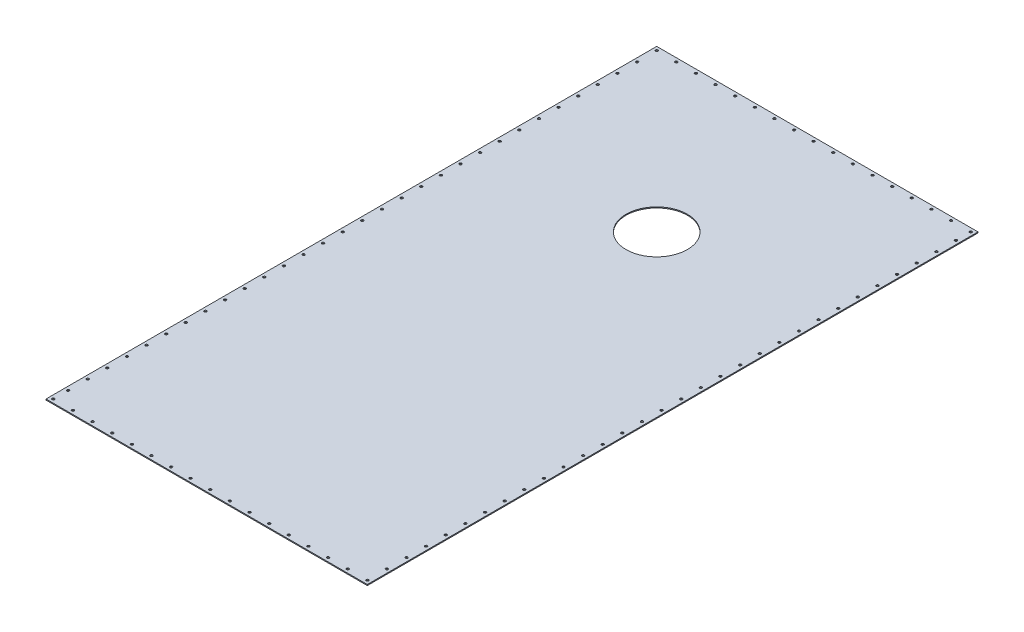
from build123d import *

# Parameters (mm, degrees)
SKETCH_1_W               = 1310
SKETCH_1_H               = 2490
EXTRUDE_1_DEPTH          = 4
PATTERN_LINEAR_1_COUNT   = 17
PATTERN_LINEAR_1_PITCH   = 80
PATTERN_CIRCULAR_1_COUNT = 2
SKETCH_4_R               = 125
CUT_EXTRUDE_1_DEPTH      = 2814.577082648
PATTERN_LINEAR_2_COUNT   = 30
PATTERN_LINEAR_2_PITCH   = 80
PATTERN_CIRCULAR_2_COUNT = 2


with BuildPart() as part:
    # 草图1 → 凸台-拉伸1 (new body)
    with BuildSketch(Plane(origin=(0, 0, 0), x_dir=(1, 0, 0), z_dir=(0, 1, 0))):
        with Locations((655, 1245)):
            Rectangle(SKETCH_1_W, SKETCH_1_H)
    extrude(amount=EXTRUDE_1_DEPTH)

    # 草图2 → Ø10.0 (10) 直径孔1 (revolve, cut)
    with BuildSketch(Plane(origin=(15, 4, -15), x_dir=(0, 0, 1), z_dir=(1, 0, 0))):
        Polygon((0, 0), (0, 13.004303095), (5, 10), (5, 0), align=None)
    hole_wizard_10_0_10_1 = revolve(axis=Axis((15, 10.35, -15), (0, -1, 0)), mode=Mode.SUBTRACT)

    # 阵列(线性)1: Ø10.0 (10) 直径孔1 ×17
    with Locations(*[(i * PATTERN_LINEAR_1_PITCH, 0, 0) for i in range(1, PATTERN_LINEAR_1_COUNT)]):
        add(hole_wizard_10_0_10_1, mode=Mode.SUBTRACT)

    # 阵列(圆周)1: Ø10.0 (10) 直径孔1 ×2 about axis
    pattern_circular_1_axis = Axis((655, 0, -1245), (0, 1, 0))
    for i in range(1, PATTERN_CIRCULAR_1_COUNT):
        add(hole_wizard_10_0_10_1.rotate(pattern_circular_1_axis, i * 360 / PATTERN_CIRCULAR_1_COUNT), mode=Mode.SUBTRACT)

    # 阵列(圆周)1 copy 1 sketch → 阵列(圆周)1 copy 1 (revolve, cut)
    with BuildSketch(Plane(origin=(1215, 4, -2475), x_dir=(0, 0, -1), z_dir=(-1, 0, 0))):
        Polygon((0, 0), (0, 13.004303095), (5, 10), (5, 0), align=None)
    revolve(axis=Axis((1215, 10.35, -2475), (0, -1, 0)), mode=Mode.SUBTRACT)

    # 阵列(圆周)1 copy 2 sketch → 阵列(圆周)1 copy 2 (revolve, cut)
    with BuildSketch(Plane(origin=(1135, 4, -2475), x_dir=(0, 0, -1), z_dir=(-1, 0, 0))):
        Polygon((0, 0), (0, 13.004303095), (5, 10), (5, 0), align=None)
    revolve(axis=Axis((1135, 10.35, -2475), (0, -1, 0)), mode=Mode.SUBTRACT)

    # 阵列(圆周)1 copy 3 sketch → 阵列(圆周)1 copy 3 (revolve, cut)
    with BuildSketch(Plane(origin=(1055, 4, -2475), x_dir=(0, 0, -1), z_dir=(-1, 0, 0))):
        Polygon((0, 0), (0, 13.004303095), (5, 10), (5, 0), align=None)
    revolve(axis=Axis((1055, 10.35, -2475), (0, -1, 0)), mode=Mode.SUBTRACT)

    # 阵列(圆周)1 copy 4 sketch → 阵列(圆周)1 copy 4 (revolve, cut)
    with BuildSketch(Plane(origin=(975, 4, -2475), x_dir=(0, 0, -1), z_dir=(-1, 0, 0))):
        Polygon((0, 0), (0, 13.004303095), (5, 10), (5, 0), align=None)
    revolve(axis=Axis((975, 10.35, -2475), (0, -1, 0)), mode=Mode.SUBTRACT)

    # 阵列(圆周)1 copy 5 sketch → 阵列(圆周)1 copy 5 (revolve, cut)
    with BuildSketch(Plane(origin=(895, 4, -2475), x_dir=(0, 0, -1), z_dir=(-1, 0, 0))):
        Polygon((0, 0), (0, 13.004303095), (5, 10), (5, 0), align=None)
    revolve(axis=Axis((895, 10.35, -2475), (0, -1, 0)), mode=Mode.SUBTRACT)

    # 阵列(圆周)1 copy 6 sketch → 阵列(圆周)1 copy 6 (revolve, cut)
    with BuildSketch(Plane(origin=(815, 4, -2475), x_dir=(0, 0, -1), z_dir=(-1, 0, 0))):
        Polygon((0, 0), (0, 13.004303095), (5, 10), (5, 0), align=None)
    revolve(axis=Axis((815, 10.35, -2475), (0, -1, 0)), mode=Mode.SUBTRACT)

    # 阵列(圆周)1 copy 7 sketch → 阵列(圆周)1 copy 7 (revolve, cut)
    with BuildSketch(Plane(origin=(735, 4, -2475), x_dir=(0, 0, -1), z_dir=(-1, 0, 0))):
        Polygon((0, 0), (0, 13.004303095), (5, 10), (5, 0), align=None)
    revolve(axis=Axis((735, 10.35, -2475), (0, -1, 0)), mode=Mode.SUBTRACT)

    # 阵列(圆周)1 copy 8 sketch → 阵列(圆周)1 copy 8 (revolve, cut)
    with BuildSketch(Plane(origin=(655, 4, -2475), x_dir=(0, 0, -1), z_dir=(-1, 0, 0))):
        Polygon((0, 0), (0, 13.004303095), (5, 10), (5, 0), align=None)
    revolve(axis=Axis((655, 10.35, -2475), (0, -1, 0)), mode=Mode.SUBTRACT)

    # 阵列(圆周)1 copy 9 sketch → 阵列(圆周)1 copy 9 (revolve, cut)
    with BuildSketch(Plane(origin=(575, 4, -2475), x_dir=(0, 0, -1), z_dir=(-1, 0, 0))):
        Polygon((0, 0), (0, 13.004303095), (5, 10), (5, 0), align=None)
    revolve(axis=Axis((575, 10.35, -2475), (0, -1, 0)), mode=Mode.SUBTRACT)

    # 阵列(圆周)1 copy 10 sketch → 阵列(圆周)1 copy 10 (revolve, cut)
    with BuildSketch(Plane(origin=(495, 4, -2475), x_dir=(0, 0, -1), z_dir=(-1, 0, 0))):
        Polygon((0, 0), (0, 13.004303095), (5, 10), (5, 0), align=None)
    revolve(axis=Axis((495, 10.35, -2475), (0, -1, 0)), mode=Mode.SUBTRACT)

    # 阵列(圆周)1 copy 11 sketch → 阵列(圆周)1 copy 11 (revolve, cut)
    with BuildSketch(Plane(origin=(415, 4, -2475), x_dir=(0, 0, -1), z_dir=(-1, 0, 0))):
        Polygon((0, 0), (0, 13.004303095), (5, 10), (5, 0), align=None)
    revolve(axis=Axis((415, 10.35, -2475), (0, -1, 0)), mode=Mode.SUBTRACT)

    # 阵列(圆周)1 copy 12 sketch → 阵列(圆周)1 copy 12 (revolve, cut)
    with BuildSketch(Plane(origin=(335, 4, -2475), x_dir=(0, 0, -1), z_dir=(-1, 0, 0))):
        Polygon((0, 0), (0, 13.004303095), (5, 10), (5, 0), align=None)
    revolve(axis=Axis((335, 10.35, -2475), (0, -1, 0)), mode=Mode.SUBTRACT)

    # 阵列(圆周)1 copy 13 sketch → 阵列(圆周)1 copy 13 (revolve, cut)
    with BuildSketch(Plane(origin=(255, 4, -2475), x_dir=(0, 0, -1), z_dir=(-1, 0, 0))):
        Polygon((0, 0), (0, 13.004303095), (5, 10), (5, 0), align=None)
    revolve(axis=Axis((255, 10.35, -2475), (0, -1, 0)), mode=Mode.SUBTRACT)

    # 阵列(圆周)1 copy 14 sketch → 阵列(圆周)1 copy 14 (revolve, cut)
    with BuildSketch(Plane(origin=(175, 4, -2475), x_dir=(0, 0, -1), z_dir=(-1, 0, 0))):
        Polygon((0, 0), (0, 13.004303095), (5, 10), (5, 0), align=None)
    revolve(axis=Axis((175, 10.35, -2475), (0, -1, 0)), mode=Mode.SUBTRACT)

    # 阵列(圆周)1 copy 15 sketch → 阵列(圆周)1 copy 15 (revolve, cut)
    with BuildSketch(Plane(origin=(95, 4, -2475), x_dir=(0, 0, -1), z_dir=(-1, 0, 0))):
        Polygon((0, 0), (0, 13.004303095), (5, 10), (5, 0), align=None)
    revolve(axis=Axis((95, 10.35, -2475), (0, -1, 0)), mode=Mode.SUBTRACT)

    # 阵列(圆周)1 copy 16 sketch → 阵列(圆周)1 copy 16 (revolve, cut)
    with BuildSketch(Plane(origin=(15, 4, -2475), x_dir=(0, 0, -1), z_dir=(-1, 0, 0))):
        Polygon((0, 0), (0, 13.004303095), (5, 10), (5, 0), align=None)
    revolve(axis=Axis((15, 10.35, -2475), (0, -1, 0)), mode=Mode.SUBTRACT)

    # 草图4 → 切除-拉伸1 (cut, through all)
    with BuildSketch(Plane(origin=(0, 4, 0), x_dir=(1, 0, 0), z_dir=(0, 1, 0))):
        with Locations(Location((655, 1835, 0), (0, 0, 270))):
            Circle(SKETCH_4_R)
    extrude(amount=-CUT_EXTRUDE_1_DEPTH, mode=Mode.SUBTRACT)

    # 草图5 → Ø10.0 (10) 直径孔2 (revolve, cut)
    with BuildSketch(Plane(origin=(15, 4, -2395), x_dir=(0, 0, 1), z_dir=(1, 0, 0))):
        Polygon((0, 0), (0, 1269.004303095), (5, 1266), (5, 0), align=None)
    hole_wizard_10_0_10_2 = revolve(axis=Axis((15, 10.35, -2395), (0, -1, 0)), mode=Mode.SUBTRACT)

    # 阵列(线性)2: Ø10.0 (10) 直径孔2 ×30
    with Locations(*[(0, 0, i * PATTERN_LINEAR_2_PITCH) for i in range(1, PATTERN_LINEAR_2_COUNT)]):
        add(hole_wizard_10_0_10_2, mode=Mode.SUBTRACT)

    # 阵列(圆周)2: Ø10.0 (10) 直径孔2 ×2 about axis
    pattern_circular_2_axis = Axis((655, 0, -1245), (0, 1, 0))
    for i in range(1, PATTERN_CIRCULAR_2_COUNT):
        add(hole_wizard_10_0_10_2.rotate(pattern_circular_2_axis, i * 360 / PATTERN_CIRCULAR_2_COUNT), mode=Mode.SUBTRACT)

    # 阵列(圆周)2 copy 1 sketch → 阵列(圆周)2 copy 1 (revolve, cut)
    with BuildSketch(Plane(origin=(1295, 4, -175), x_dir=(0, 0, -1), z_dir=(-1, 0, 0))):
        Polygon((0, 0), (0, 1269.004303095), (5, 1266), (5, 0), align=None)
    revolve(axis=Axis((1295, 10.35, -175), (0, -1, 0)), mode=Mode.SUBTRACT)

    # 阵列(圆周)2 copy 2 sketch → 阵列(圆周)2 copy 2 (revolve, cut)
    with BuildSketch(Plane(origin=(1295, 4, -255), x_dir=(0, 0, -1), z_dir=(-1, 0, 0))):
        Polygon((0, 0), (0, 1269.004303095), (5, 1266), (5, 0), align=None)
    revolve(axis=Axis((1295, 10.35, -255), (0, -1, 0)), mode=Mode.SUBTRACT)

    # 阵列(圆周)2 copy 3 sketch → 阵列(圆周)2 copy 3 (revolve, cut)
    with BuildSketch(Plane(origin=(1295, 4, -335), x_dir=(0, 0, -1), z_dir=(-1, 0, 0))):
        Polygon((0, 0), (0, 1269.004303095), (5, 1266), (5, 0), align=None)
    revolve(axis=Axis((1295, 10.35, -335), (0, -1, 0)), mode=Mode.SUBTRACT)

    # 阵列(圆周)2 copy 4 sketch → 阵列(圆周)2 copy 4 (revolve, cut)
    with BuildSketch(Plane(origin=(1295, 4, -415), x_dir=(0, 0, -1), z_dir=(-1, 0, 0))):
        Polygon((0, 0), (0, 1269.004303095), (5, 1266), (5, 0), align=None)
    revolve(axis=Axis((1295, 10.35, -415), (0, -1, 0)), mode=Mode.SUBTRACT)

    # 阵列(圆周)2 copy 5 sketch → 阵列(圆周)2 copy 5 (revolve, cut)
    with BuildSketch(Plane(origin=(1295, 4, -495), x_dir=(0, 0, -1), z_dir=(-1, 0, 0))):
        Polygon((0, 0), (0, 1269.004303095), (5, 1266), (5, 0), align=None)
    revolve(axis=Axis((1295, 10.35, -495), (0, -1, 0)), mode=Mode.SUBTRACT)

    # 阵列(圆周)2 copy 6 sketch → 阵列(圆周)2 copy 6 (revolve, cut)
    with BuildSketch(Plane(origin=(1295, 4, -575), x_dir=(0, 0, -1), z_dir=(-1, 0, 0))):
        Polygon((0, 0), (0, 1269.004303095), (5, 1266), (5, 0), align=None)
    revolve(axis=Axis((1295, 10.35, -575), (0, -1, 0)), mode=Mode.SUBTRACT)

    # 阵列(圆周)2 copy 7 sketch → 阵列(圆周)2 copy 7 (revolve, cut)
    with BuildSketch(Plane(origin=(1295, 4, -655), x_dir=(0, 0, -1), z_dir=(-1, 0, 0))):
        Polygon((0, 0), (0, 1269.004303095), (5, 1266), (5, 0), align=None)
    revolve(axis=Axis((1295, 10.35, -655), (0, -1, 0)), mode=Mode.SUBTRACT)

    # 阵列(圆周)2 copy 8 sketch → 阵列(圆周)2 copy 8 (revolve, cut)
    with BuildSketch(Plane(origin=(1295, 4, -735), x_dir=(0, 0, -1), z_dir=(-1, 0, 0))):
        Polygon((0, 0), (0, 1269.004303095), (5, 1266), (5, 0), align=None)
    revolve(axis=Axis((1295, 10.35, -735), (0, -1, 0)), mode=Mode.SUBTRACT)

    # 阵列(圆周)2 copy 9 sketch → 阵列(圆周)2 copy 9 (revolve, cut)
    with BuildSketch(Plane(origin=(1295, 4, -815), x_dir=(0, 0, -1), z_dir=(-1, 0, 0))):
        Polygon((0, 0), (0, 1269.004303095), (5, 1266), (5, 0), align=None)
    revolve(axis=Axis((1295, 10.35, -815), (0, -1, 0)), mode=Mode.SUBTRACT)

    # 阵列(圆周)2 copy 10 sketch → 阵列(圆周)2 copy 10 (revolve, cut)
    with BuildSketch(Plane(origin=(1295, 4, -895), x_dir=(0, 0, -1), z_dir=(-1, 0, 0))):
        Polygon((0, 0), (0, 1269.004303095), (5, 1266), (5, 0), align=None)
    revolve(axis=Axis((1295, 10.35, -895), (0, -1, 0)), mode=Mode.SUBTRACT)

    # 阵列(圆周)2 copy 11 sketch → 阵列(圆周)2 copy 11 (revolve, cut)
    with BuildSketch(Plane(origin=(1295, 4, -975), x_dir=(0, 0, -1), z_dir=(-1, 0, 0))):
        Polygon((0, 0), (0, 1269.004303095), (5, 1266), (5, 0), align=None)
    revolve(axis=Axis((1295, 10.35, -975), (0, -1, 0)), mode=Mode.SUBTRACT)

    # 阵列(圆周)2 copy 12 sketch → 阵列(圆周)2 copy 12 (revolve, cut)
    with BuildSketch(Plane(origin=(1295, 4, -1055), x_dir=(0, 0, -1), z_dir=(-1, 0, 0))):
        Polygon((0, 0), (0, 1269.004303095), (5, 1266), (5, 0), align=None)
    revolve(axis=Axis((1295, 10.35, -1055), (0, -1, 0)), mode=Mode.SUBTRACT)

    # 阵列(圆周)2 copy 13 sketch → 阵列(圆周)2 copy 13 (revolve, cut)
    with BuildSketch(Plane(origin=(1295, 4, -1135), x_dir=(0, 0, -1), z_dir=(-1, 0, 0))):
        Polygon((0, 0), (0, 1269.004303095), (5, 1266), (5, 0), align=None)
    revolve(axis=Axis((1295, 10.35, -1135), (0, -1, 0)), mode=Mode.SUBTRACT)

    # 阵列(圆周)2 copy 14 sketch → 阵列(圆周)2 copy 14 (revolve, cut)
    with BuildSketch(Plane(origin=(1295, 4, -1215), x_dir=(0, 0, -1), z_dir=(-1, 0, 0))):
        Polygon((0, 0), (0, 1269.004303095), (5, 1266), (5, 0), align=None)
    revolve(axis=Axis((1295, 10.35, -1215), (0, -1, 0)), mode=Mode.SUBTRACT)

    # 阵列(圆周)2 copy 15 sketch → 阵列(圆周)2 copy 15 (revolve, cut)
    with BuildSketch(Plane(origin=(1295, 4, -1295), x_dir=(0, 0, -1), z_dir=(-1, 0, 0))):
        Polygon((0, 0), (0, 1269.004303095), (5, 1266), (5, 0), align=None)
    revolve(axis=Axis((1295, 10.35, -1295), (0, -1, 0)), mode=Mode.SUBTRACT)

    # 阵列(圆周)2 copy 16 sketch → 阵列(圆周)2 copy 16 (revolve, cut)
    with BuildSketch(Plane(origin=(1295, 4, -1375), x_dir=(0, 0, -1), z_dir=(-1, 0, 0))):
        Polygon((0, 0), (0, 1269.004303095), (5, 1266), (5, 0), align=None)
    revolve(axis=Axis((1295, 10.35, -1375), (0, -1, 0)), mode=Mode.SUBTRACT)

    # 阵列(圆周)2 copy 17 sketch → 阵列(圆周)2 copy 17 (revolve, cut)
    with BuildSketch(Plane(origin=(1295, 4, -1455), x_dir=(0, 0, -1), z_dir=(-1, 0, 0))):
        Polygon((0, 0), (0, 1269.004303095), (5, 1266), (5, 0), align=None)
    revolve(axis=Axis((1295, 10.35, -1455), (0, -1, 0)), mode=Mode.SUBTRACT)

    # 阵列(圆周)2 copy 18 sketch → 阵列(圆周)2 copy 18 (revolve, cut)
    with BuildSketch(Plane(origin=(1295, 4, -1535), x_dir=(0, 0, -1), z_dir=(-1, 0, 0))):
        Polygon((0, 0), (0, 1269.004303095), (5, 1266), (5, 0), align=None)
    revolve(axis=Axis((1295, 10.35, -1535), (0, -1, 0)), mode=Mode.SUBTRACT)

    # 阵列(圆周)2 copy 19 sketch → 阵列(圆周)2 copy 19 (revolve, cut)
    with BuildSketch(Plane(origin=(1295, 4, -1615), x_dir=(0, 0, -1), z_dir=(-1, 0, 0))):
        Polygon((0, 0), (0, 1269.004303095), (5, 1266), (5, 0), align=None)
    revolve(axis=Axis((1295, 10.35, -1615), (0, -1, 0)), mode=Mode.SUBTRACT)

    # 阵列(圆周)2 copy 20 sketch → 阵列(圆周)2 copy 20 (revolve, cut)
    with BuildSketch(Plane(origin=(1295, 4, -1695), x_dir=(0, 0, -1), z_dir=(-1, 0, 0))):
        Polygon((0, 0), (0, 1269.004303095), (5, 1266), (5, 0), align=None)
    revolve(axis=Axis((1295, 10.35, -1695), (0, -1, 0)), mode=Mode.SUBTRACT)

    # 阵列(圆周)2 copy 21 sketch → 阵列(圆周)2 copy 21 (revolve, cut)
    with BuildSketch(Plane(origin=(1295, 4, -1775), x_dir=(0, 0, -1), z_dir=(-1, 0, 0))):
        Polygon((0, 0), (0, 1269.004303095), (5, 1266), (5, 0), align=None)
    revolve(axis=Axis((1295, 10.35, -1775), (0, -1, 0)), mode=Mode.SUBTRACT)

    # 阵列(圆周)2 copy 22 sketch → 阵列(圆周)2 copy 22 (revolve, cut)
    with BuildSketch(Plane(origin=(1295, 4, -1855), x_dir=(0, 0, -1), z_dir=(-1, 0, 0))):
        Polygon((0, 0), (0, 1269.004303095), (5, 1266), (5, 0), align=None)
    revolve(axis=Axis((1295, 10.35, -1855), (0, -1, 0)), mode=Mode.SUBTRACT)

    # 阵列(圆周)2 copy 23 sketch → 阵列(圆周)2 copy 23 (revolve, cut)
    with BuildSketch(Plane(origin=(1295, 4, -1935), x_dir=(0, 0, -1), z_dir=(-1, 0, 0))):
        Polygon((0, 0), (0, 1269.004303095), (5, 1266), (5, 0), align=None)
    revolve(axis=Axis((1295, 10.35, -1935), (0, -1, 0)), mode=Mode.SUBTRACT)

    # 阵列(圆周)2 copy 24 sketch → 阵列(圆周)2 copy 24 (revolve, cut)
    with BuildSketch(Plane(origin=(1295, 4, -2015), x_dir=(0, 0, -1), z_dir=(-1, 0, 0))):
        Polygon((0, 0), (0, 1269.004303095), (5, 1266), (5, 0), align=None)
    revolve(axis=Axis((1295, 10.35, -2015), (0, -1, 0)), mode=Mode.SUBTRACT)

    # 阵列(圆周)2 copy 25 sketch → 阵列(圆周)2 copy 25 (revolve, cut)
    with BuildSketch(Plane(origin=(1295, 4, -2095), x_dir=(0, 0, -1), z_dir=(-1, 0, 0))):
        Polygon((0, 0), (0, 1269.004303095), (5, 1266), (5, 0), align=None)
    revolve(axis=Axis((1295, 10.35, -2095), (0, -1, 0)), mode=Mode.SUBTRACT)

    # 阵列(圆周)2 copy 26 sketch → 阵列(圆周)2 copy 26 (revolve, cut)
    with BuildSketch(Plane(origin=(1295, 4, -2175), x_dir=(0, 0, -1), z_dir=(-1, 0, 0))):
        Polygon((0, 0), (0, 1269.004303095), (5, 1266), (5, 0), align=None)
    revolve(axis=Axis((1295, 10.35, -2175), (0, -1, 0)), mode=Mode.SUBTRACT)

    # 阵列(圆周)2 copy 27 sketch → 阵列(圆周)2 copy 27 (revolve, cut)
    with BuildSketch(Plane(origin=(1295, 4, -2255), x_dir=(0, 0, -1), z_dir=(-1, 0, 0))):
        Polygon((0, 0), (0, 1269.004303095), (5, 1266), (5, 0), align=None)
    revolve(axis=Axis((1295, 10.35, -2255), (0, -1, 0)), mode=Mode.SUBTRACT)

    # 阵列(圆周)2 copy 28 sketch → 阵列(圆周)2 copy 28 (revolve, cut)
    with BuildSketch(Plane(origin=(1295, 4, -2335), x_dir=(0, 0, -1), z_dir=(-1, 0, 0))):
        Polygon((0, 0), (0, 1269.004303095), (5, 1266), (5, 0), align=None)
    revolve(axis=Axis((1295, 10.35, -2335), (0, -1, 0)), mode=Mode.SUBTRACT)

    # 阵列(圆周)2 copy 29 sketch → 阵列(圆周)2 copy 29 (revolve, cut)
    with BuildSketch(Plane(origin=(1295, 4, -2415), x_dir=(0, 0, -1), z_dir=(-1, 0, 0))):
        Polygon((0, 0), (0, 1269.004303095), (5, 1266), (5, 0), align=None)
    revolve(axis=Axis((1295, 10.35, -2415), (0, -1, 0)), mode=Mode.SUBTRACT)


solid = part.part
